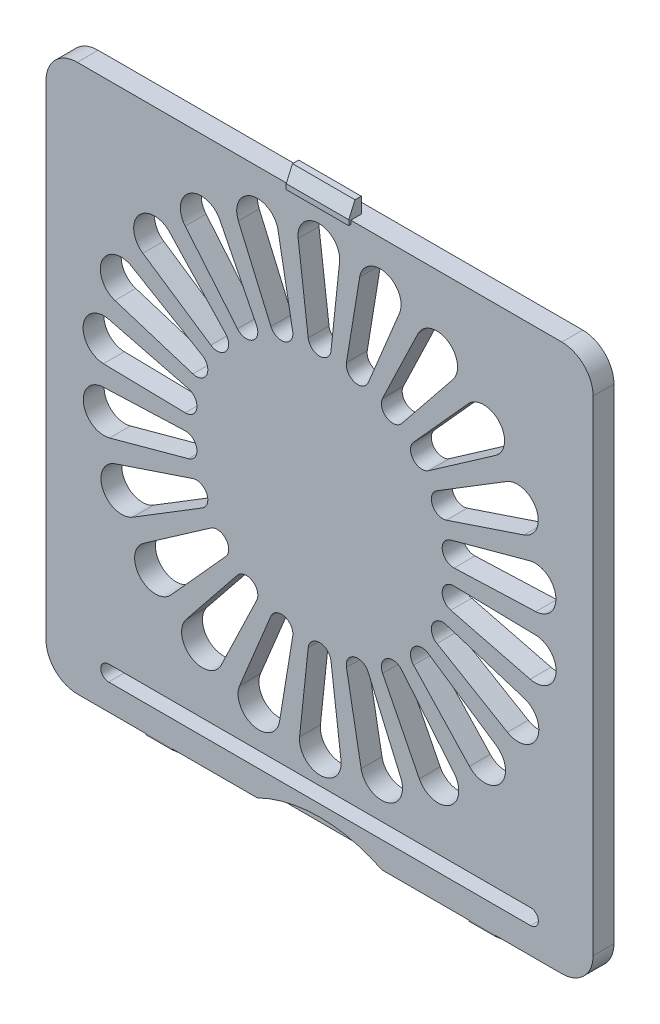
from build123d import *

# Parameters (mm, degrees)
BOSS_EXTRUDE1_DEPTH = 2
CUT_EXTRUDE1_DEPTH  = 12
CUT_EXTRUDE2_START  = -1
SKETCH3_R           = 13.5
CUT_EXTRUDE2_DEPTH  = 1
BOSS_EXTRUDE2_START = 14.25
BOSS_EXTRUDE2_DEPTH = 2.5
BOSS_EXTRUDE3_DEPTH = 3


with BuildPart() as part:
    # Sketch1 → Boss-Extrude1 (new body)
    with BuildSketch(Plane.XY):
        with BuildLine():
            Line((-23.25, 26.25), (23.25, 26.25))
            ThreePointArc((23.25, 26.25), (25.371320344, 25.371320344), (26.25, 23.25))
            Line((26.25, 23.25), (26.25, -23.25))
            ThreePointArc((26.25, -23.25), (25.371320344, -25.371320344), (23.25, -26.25))
            Line((23.25, -26.25), (-23.25, -26.25))
            ThreePointArc((-23.25, -26.25), (-25.371320344, -25.371320344), (-26.25, -23.25))
            Line((-26.25, -23.25), (-26.25, 23.25))
            ThreePointArc((-26.25, 23.25), (-25.371320344, 25.371320344), (-23.25, 26.25))
        make_face()
    extrude(amount=BOSS_EXTRUDE1_DEPTH)

    # Sketch2 → Cut-Extrude1 (cut)
    with BuildSketch(Plane.XY.offset(2)):
        with BuildLine():
            Line((-20.25, -22.25), (20.25, -22.25))
            ThreePointArc((20.25, -22.25), (21, -23), (20.25, -23.75))
            Line((20.25, -23.75), (-20.25, -23.75))
            ThreePointArc((-20.25, -23.75), (-21, -23), (-20.25, -22.25))
        make_face()
        with BuildLine():
            Line((-2.05533329, 22.204447747), (-1.091677831, 14.414946261))
            ThreePointArc((-1.091677831, 14.414946261), (0.009811123, 13.450043755), (1.093913188, 14.434440766))
            Line((1.093913188, 14.434440766), (1.918468564, 22.239892302))
            ThreePointArc((1.918468564, 22.239892302), (-0.088302912, 24.449920446), (-2.05533329, 22.204447747))
        make_face()
        with BuildLine():
            Line((3.846952523, 21.94685179), (2.577016995, 14.20138673))
            ThreePointArc((2.577016995, 14.20138673), (3.362043457, 12.965244255), (4.679568458, 13.604339425))
            Line((4.679568458, 13.604339425), (7.669773366, 20.861311235))
            ThreePointArc((7.669773366, 20.861311235), (6.366927115, 23.54719057), (3.846952523, 21.94685179))
        make_face()
        with BuildLine():
            Line((9.437581122, 20.036824206), (6.036937231, 12.962887087))
            ThreePointArc((6.036937231, 12.962887087), (6.441903025, 11.555649556), (7.886112922, 11.797667193))
            Line((7.886112922, 11.797667193), (12.799718744, 17.91824258))
            ThreePointArc((12.799718744, 17.91824258), (12.306346573, 20.862379135), (9.437581122, 20.036824206))
        make_face()
        with BuildLine():
            Line((14.263633026, 16.62910407), (9.007780715, 10.799783207))
            ThreePointArc((9.007780715, 10.799783207), (8.999877922, 9.335456635), (10.453771418, 9.16078991))
            Line((10.453771418, 9.16078991), (16.892707032, 13.649116258))
            ThreePointArc((16.892707032, 13.649116258), (17.24877902, 16.612993599), (14.263633026, 16.62910407))
        make_face()
        with BuildLine():
            Line((17.934130212, 11.999764601), (11.248867377, 7.887316902))
            ThreePointArc((11.248867377, 7.887316902), (10.828736233, 6.484532319), (12.174527524, 5.907331692))
            Line((12.174527524, 5.907331692), (19.617148662, 8.399791492))
            ThreePointArc((19.617148662, 8.399791492), (20.793817974, 11.143293904), (17.934130212, 11.999764601))
        make_face()
        with BuildLine():
            Line((20.151710825, 6.523847352), (12.578637704, 4.461438872))
            ThreePointArc((12.578637704, 4.461438872), (11.780314736, 3.233841542), (12.908975815, 2.300868375))
            Line((12.908975815, 2.300868375), (20.752325574, 2.595537357))
            ThreePointArc((20.752325574, 2.595537357), (22.65426546, 4.89640259), (20.151710825, 6.523847352))
        make_face()
        with BuildLine():
            Line((20.736719675, 0.64497857), (12.889361612, 0.799693379))
            ThreePointArc((12.889361612, 0.799693379), (11.777522199, -0.153264063), (12.597615658, -1.366425833))
            Line((12.597615658, -1.366425833), (20.206272487, -3.293419997))
            ThreePointArc((20.206272487, -3.293419997), (22.67939909, -1.621594359), (20.736719675, 0.64497857))
        make_face()
        with BuildLine():
            Line((19.641762823, -5.160570757), (12.155866098, -2.801266734))
            ThreePointArc((12.155866098, -2.801266734), (10.820584857, -3.402381343), (11.265671602, -4.797448565))
            Line((11.265671602, -4.797448565), (18.023227375, -8.789992267))
            ThreePointArc((18.023227375, -8.789992267), (20.867182684, -7.882647596), (19.641762823, -5.160570757))
        make_face()
        with BuildLine():
            Line((16.95554716, -10.422469552), (10.437574607, -6.049713094))
            ThreePointArc((10.437574607, -6.049713094), (8.987028083, -6.250286139), (9.021049831, -7.714238763))
            Line((9.021049831, -7.714238763), (14.380047569, -13.448879859))
            ThreePointArc((14.380047569, -13.448879859), (17.36443124, -13.379523823), (16.95554716, -10.422469552))
        make_face()
        with BuildLine():
            Line((12.895693906, -14.714430066), (7.873692895, -8.682475896))
            ThreePointArc((7.873692895, -8.682475896), (6.425395741, -8.466258143), (6.045596254, -9.880495433))
            Line((6.045596254, -9.880495433), (9.57188183, -16.892647405))
            ThreePointArc((9.57188183, -16.892647405), (12.454916846, -17.666898819), (12.895693906, -14.714430066))
        make_face()
        with BuildLine():
            Line((7.791108224, -17.688743184), (4.671931412, -10.486264357))
            ThreePointArc((4.671931412, -10.486264357), (3.34321605, -9.870772481), (2.580364423, -11.120721344))
            Line((2.580364423, -11.120721344), (3.988259152, -18.842301342))
            ThreePointArc((3.988259152, -18.842301342), (6.536379162, -20.397434959), (7.791108224, -17.688743184))
        make_face()
        with BuildLine():
            Line((2.05533329, -19.104447747), (1.091677831, -11.314946261))
            ThreePointArc((1.091677831, -11.314946261), (-0.009811123, -10.350043755), (-1.093913188, -11.334440766))
            Line((-1.093913188, -11.334440766), (-1.918468564, -19.139892302))
            ThreePointArc((-1.918468564, -19.139892302), (0.088302912, -21.349920446), (2.05533329, -19.104447747))
        make_face()
        with BuildLine():
            Line((-3.846952523, -18.84685179), (-2.577016995, -11.10138673))
            ThreePointArc((-2.577016995, -11.10138673), (-3.362043457, -9.865244255), (-4.679568458, -10.504339425))
            Line((-4.679568458, -10.504339425), (-7.669773366, -17.761311235))
            ThreePointArc((-7.669773366, -17.761311235), (-6.366927115, -20.44719057), (-3.846952523, -18.84685179))
        make_face()
        with BuildLine():
            Line((-9.437581122, -16.936824206), (-6.036937231, -9.862887087))
            ThreePointArc((-6.036937231, -9.862887087), (-6.441903025, -8.455649556), (-7.886112922, -8.697667193))
            Line((-7.886112922, -8.697667193), (-12.799718744, -14.81824258))
            ThreePointArc((-12.799718744, -14.81824258), (-12.306346573, -17.762379135), (-9.437581122, -16.936824206))
        make_face()
        with BuildLine():
            Line((-14.263633026, -13.52910407), (-9.007780715, -7.699783207))
            ThreePointArc((-9.007780715, -7.699783207), (-8.999877922, -6.235456635), (-10.453771418, -6.06078991))
            Line((-10.453771418, -6.06078991), (-16.892707032, -10.549116258))
            ThreePointArc((-16.892707032, -10.549116258), (-17.24877902, -13.512993599), (-14.263633026, -13.52910407))
        make_face()
        with BuildLine():
            Line((-17.934130212, -8.899764601), (-11.248867377, -4.787316902))
            ThreePointArc((-11.248867377, -4.787316902), (-10.828736233, -3.384532319), (-12.174527524, -2.807331692))
            Line((-12.174527524, -2.807331692), (-19.617148662, -5.299791492))
            ThreePointArc((-19.617148662, -5.299791492), (-20.793817974, -8.043293904), (-17.934130212, -8.899764601))
        make_face()
        with BuildLine():
            Line((-20.151710825, -3.423847352), (-12.578637704, -1.361438872))
            ThreePointArc((-12.578637704, -1.361438872), (-11.780314736, -0.133841542), (-12.908975815, 0.799131625))
            Line((-12.908975815, 0.799131625), (-20.752325574, 0.504462643))
            ThreePointArc((-20.752325574, 0.504462643), (-22.65426546, -1.79640259), (-20.151710825, -3.423847352))
        make_face()
        with BuildLine():
            Line((-20.736719675, 2.45502143), (-12.889361612, 2.300306621))
            ThreePointArc((-12.889361612, 2.300306621), (-11.777522199, 3.253264063), (-12.597615658, 4.466425833))
            Line((-12.597615658, 4.466425833), (-20.206272487, 6.393419997))
            ThreePointArc((-20.206272487, 6.393419997), (-22.67939909, 4.721594359), (-20.736719675, 2.45502143))
        make_face()
        with BuildLine():
            Line((-19.641762823, 8.260570757), (-12.155866098, 5.901266734))
            ThreePointArc((-12.155866098, 5.901266734), (-10.820584857, 6.502381343), (-11.265671602, 7.897448565))
            Line((-11.265671602, 7.897448565), (-18.023227375, 11.889992267))
            ThreePointArc((-18.023227375, 11.889992267), (-20.867182684, 10.982647596), (-19.641762823, 8.260570757))
        make_face()
        with BuildLine():
            Line((-16.95554716, 13.522469552), (-10.437574607, 9.149713094))
            ThreePointArc((-10.437574607, 9.149713094), (-8.987028083, 9.350286139), (-9.021049831, 10.814238763))
            Line((-9.021049831, 10.814238763), (-14.380047569, 16.548879859))
            ThreePointArc((-14.380047569, 16.548879859), (-17.36443124, 16.479523823), (-16.95554716, 13.522469552))
        make_face()
        with BuildLine():
            Line((-12.895693906, 17.814430066), (-7.873692895, 11.782475896))
            ThreePointArc((-7.873692895, 11.782475896), (-6.425395741, 11.566258143), (-6.045596254, 12.980495433))
            Line((-6.045596254, 12.980495433), (-9.57188183, 19.992647405))
            ThreePointArc((-9.57188183, 19.992647405), (-12.454916846, 20.766898819), (-12.895693906, 17.814430066))
        make_face()
        with BuildLine():
            Line((-7.791108224, 20.788743184), (-4.671931412, 13.586264357))
            ThreePointArc((-4.671931412, 13.586264357), (-3.34321605, 12.970772481), (-2.580364423, 14.220721344))
            Line((-2.580364423, 14.220721344), (-3.988259152, 21.942301342))
            ThreePointArc((-3.988259152, 21.942301342), (-6.536379162, 23.497434959), (-7.791108224, 20.788743184))
        make_face()
    extrude(amount=-CUT_EXTRUDE1_DEPTH, mode=Mode.SUBTRACT)

    # Sketch3 → Cut-Extrude2 (cut)
    with BuildSketch(Plane(origin=(0, 0, 0), x_dir=(-1, 0, 0), z_dir=(0, 0, -1)).offset(CUT_EXTRUDE2_START)):
        with Locations((0, -38.352973417)):
            Circle(SKETCH3_R)
    extrude(amount=-CUT_EXTRUDE2_DEPTH, mode=Mode.SUBTRACT)

    # Sketch4 → Boss-Extrude2 (add)
    with BuildSketch(Plane(origin=(0, 0, 0), x_dir=(0, 0, -1), z_dir=(1, 0, 0)).offset(BOSS_EXTRUDE2_START)):
        Polygon((-1, -26.25), (-1, -27), (-1.25, -27), (-1.892304423, -26.45), (-1.892304423, -26.25), align=None)
    boss_extrude2 = extrude(amount=BOSS_EXTRUDE2_DEPTH)

    # Mirror3: Boss-Extrude2 across plane
    add(boss_extrude2.mirror(Plane(origin=(0, 0, 0), x_dir=(0, 0, 1), z_dir=(1, 0, 0))))

    # Sketch5 → Boss-Extrude3 (add, symmetric)
    with BuildSketch(Plane(origin=(0, 0, 0), x_dir=(0, 0, -1), z_dir=(1, 0, 0))):
        Polygon((-1, 26.25), (-1, 27.75), (-1.6, 27.75), (-2.2, 26.392012559), (-2.2, 25.892012559), (-1, 25.892012559), align=None)
    extrude(amount=BOSS_EXTRUDE3_DEPTH, both=True)


solid = part.part
